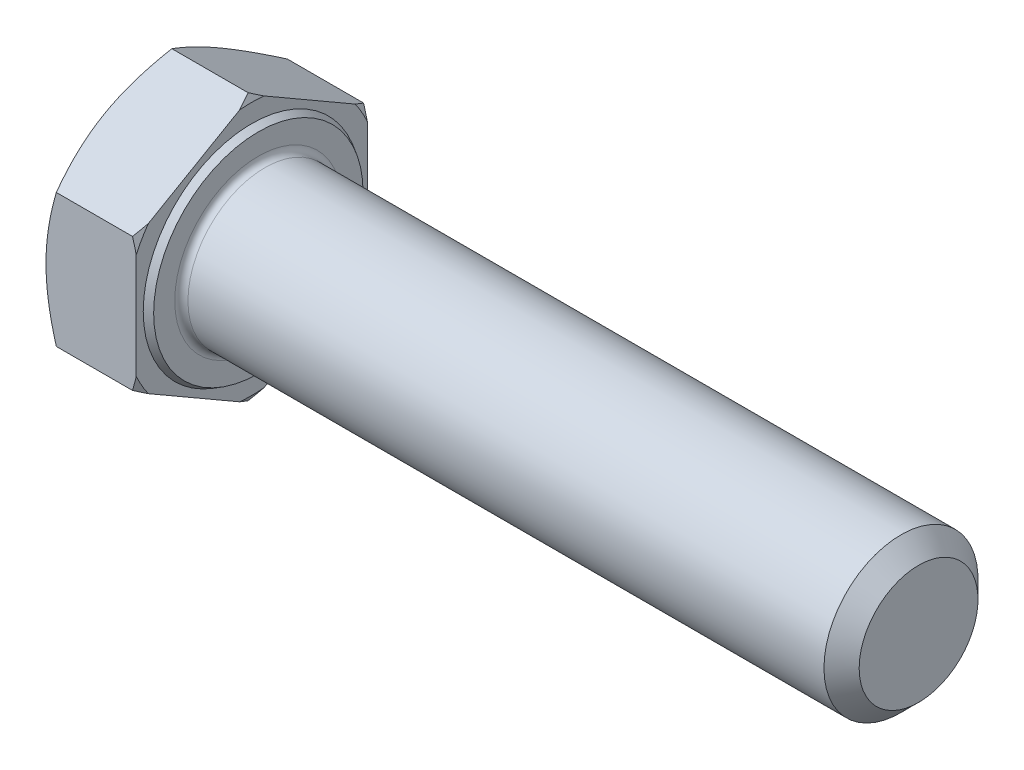
from build123d import *

# Parameters (mm, degrees)
BOSS_EXTRUDE_DEPTH = 8.8
CHAMFER_2_SIZE     = 1.6


with BuildPart() as part:
    # Sketch1 → Boss-Extrude (new body)
    with BuildSketch(Plane(origin=(0, 0, 0), x_dir=(0, 0, -1), z_dir=(1, 0, 0))):
        Polygon((10.5, 6.062177826), (10.5, -6.062177826), (0, -12.124355653), (-10.5, -6.062177826), (-10.5, 6.062177826), (0, 12.124355653), align=None)
    extrude(amount=BOSS_EXTRUDE_DEPTH)

    # Sketch2 → Boss-Revolve1 (revolve)
    with BuildSketch(Plane.XY, mode=Mode.PRIVATE) as boss_revolve1_sk:
        Polygon((0, 0), (68.8, 0), (68.8, 5.268), (68.8, 7), (8.8, 7), (0, 7), align=None)
    revolve(boss_revolve1_sk.sketch.rotate(Axis((0, 0, 0), (-1, 0, 0)), 90), axis=Axis((0, 0, 0), (-1, 0, 0)))

    # Sketch3 → Cut-Revolve1 (revolve, cut)
    with BuildSketch(Plane.XY):
        Polygon((0, 10.5), (3.824573519, 17.124355653), (3.824573519, 22.124355653), (-10, 22.124355653), (-10, 10.5), align=None)
    revolve(axis=Axis((0, 0, 0), (1, 0, 0)), mode=Mode.SUBTRACT)

    # Sketch5 → Cut-Revolve2 (revolve, cut)
    with BuildSketch(Plane.XY):
        Polygon((8.8, 10.5), (4.975426481, 17.124355653), (4.975426481, 22.124355653), (14.975426481, 22.124355653), (14.975426481, 10.5), align=None)
    revolve(axis=Axis((0, 0, 0), (1, 0, 0)), mode=Mode.SUBTRACT)

    # Sketch4 → Cut-Revolve3 (revolve, cut)
    with BuildSketch(Plane.XY, mode=Mode.PRIVATE) as cut_revolve3_sk:
        Polygon((8.8, 9.517264973), (8.2, 9.863675135), (8.2, 22.124355653), (8.8, 22.124355653), align=None)
    revolve(cut_revolve3_sk.sketch.rotate(Axis((0, 0, 0), (1, 0, 0)), 90), axis=Axis((0, 0, 0), (1, 0, 0)), mode=Mode.SUBTRACT)

    # Chamfer 2
    chamfer_2_edges = [part.edges().sort_by_distance(p)[0] for p in [
        (68.8, 0, 7),
    ]]
    chamfer(chamfer_2_edges, length=CHAMFER_2_SIZE)

    # Sketch9 → Revolve1 (revolve)
    with BuildSketch(Plane.XY, mode=Mode.PRIVATE) as revolve1_sk:
        with BuildLine():
            Line((8.8, 7.6), (8.8, 7))
            Line((8.8, 7), (9.4, 7))
            ThreePointArc((9.4, 7), (8.975735931, 7.175735931), (8.8, 7.6))
        make_face()
    revolve(revolve1_sk.sketch.rotate(Axis((0, 0, 0), (1, 0, 0)), 90), axis=Axis((0, 0, 0), (1, 0, 0)))


solid = part.part
